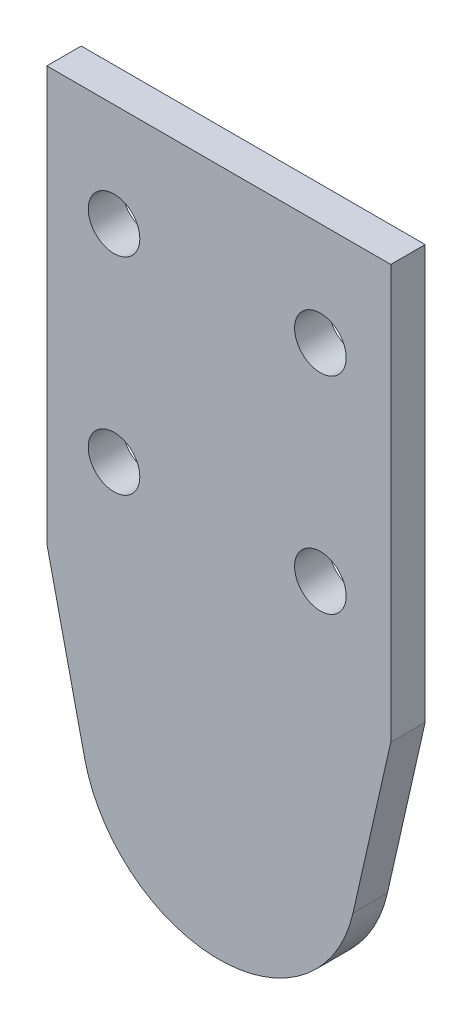
SolidWorks part; units mm, degrees
ref_plane "前视基准面" through (0, 0, 0) normal (0, 0, 1) x (1, 0, 0)
ref_plane "上视基准面" through (0, 0, 0) normal (0, 1, 0) x (1, 0, 0)
ref_plane "右视基准面" through (0, 0, 0) normal (1, 0, 0) x (0, 0, -1)
sketch "草图1" plane through (0, 0, 0) normal (0, 0, 1) x (1, 0, 0)
  line L0 (0, 0) -> (90, 0)
  line L3 (0, 0) -> (5.0194, -161.2446)
  line L4 (90, 0) -> (84.9806, -161.2446)
  arc A0 (5.0194, -161.2446) -> (84.9806, -161.2446) centre (45, -160) ccw
  circle A1 centre (45, -160) radius 20
extrude "凸台-拉伸1" add sketch "草图1" along normal blind 10
sketch "草图2" plane through (0, 0, 10) normal (0, 0, 1) x (1, 0, 0)
  line L0 (0, 0) -> (0, -30)
  line L1 (14.5331, -30) -> (22.0331, -30)
  line L2 (74.5331, -30) -> (74.5331, -90)
  line L3 (74.5331, -90) -> (14.5331, -90)
  line L4 (14.5331, -90) -> (14.5331, -30)
  line L5 (0, -30) -> (22.0331, -30)
  line L6 (84.9806, -161.2446) -> (90, 0) construction
  line L9 (67.0331, -30) -> (74.5331, -30)
  line L10 (67.0331, -30) -> (89.0661, -30)
  circle A0 centre (14.5331, -30) radius 7.5
  circle A1 centre (74.5331, -30) radius 7.5
  circle A2 centre (74.5331, -90) radius 7.5
  circle A3 centre (14.5331, -90) radius 7.5
extrude "切除-拉伸1" cut sketch "草图2" against normal blind 10 contours L1 A0 L5 | L4 A0 L1 | L5 A0 L4 | L10 A1 L9 | L2 A1 L10 | L9 A1 L2 | L3 A2 L2 | L2 A2 L3 | L3 A3 L4 | L4 A3 L3
sketch "草图3" plane through (0, 0, 10) normal (0, 0, 1) x (1, 0, 0)
  line L0 (0, 0) -> (0, -120)
  line L1 (90, 0) -> (90, -120)
  line L2 (90, -120) -> (84.7241, -164.6897)
  line L3 (0, -120) -> (5.2759, -164.6897)
  line L6 (0, 0) -> (5.0194, -161.2446)
  line L7 (0, 0) -> (5.0194, -161.2446)
  line L9 (84.9806, -161.2446) -> (90, 0)
  line L10 (84.9806, -161.2446) -> (90, 0)
  arc A0 (84.7241, -164.6897) -> (5.2759, -164.6897) centre (45, -160) ccw
  line M5 (0, 0) -> (5.0194, -161.2446)
  arc M6 (5.0194, -161.2446) -> (84.9806, -161.2446) centre (45, -160) ccw
  line M7 (84.9806, -161.2446) -> (90, 0)
  dimension "D1" = 0
  dimension "D2" = 0
extrude "凸台-拉伸4" add sketch "草图3" against normal blind 10 contours L2 L1 M7 M6 | L0 L3 M6 M5
sketch "草图4" plane through (0, 0, 0) normal (0, 0, -1) x (-1, 0, 0)
  line L0 (-90, 0) -> (-95, 0)
  line L1 (0, 0) -> (5, 0)
  line L2 (5, 0) -> (5, -120.2941)
  line L3 (-95, 0) -> (-95, -120.2941)
  line L14 (-0.3103, -165.2759) -> (5, -120.2941)
  line L15 (5, -120.2941) -> (5, 5)
  line L16 (5, 5) -> (-95, 5)
  line L17 (-95, 5) -> (-95, -120.2941)
  line L18 (-95, -120.2941) -> (-89.6897, -165.2759)
  line L19 (-95, -120.2941) -> (-84.013, -168.8311)
  line L20 (5, -120.2941) -> (5, 0)
  line L21 (5, -120.2941) -> (-5.987, -168.8311)
  line L22 (-95, 0) -> (-95, -120.2941)
  line L28 (-5.2759, -164.6897) -> (0, -120)
  line L29 (0, -120) -> (0, 0)
  line L30 (0, 0) -> (-90, 0)
  line L31 (-90, 0) -> (-90, -120)
  line L32 (-90, -120) -> (-84.7241, -164.6897)
  line L33 (-5.2759, -164.6897) -> (0, -120)
  line L34 (0, -120) -> (0, 0)
  line L35 (0, 0) -> (-90, 0)
  line L36 (-90, 0) -> (-90, -120)
  line L37 (-90, -120) -> (-84.7241, -164.6897)
  arc A2 (-89.6897, -165.2759) -> (-0.3103, -165.2759) centre (-45, -160) ccw
  arc A3 (-5.987, -168.8311) -> (-5.2759, -164.6897) centre (-45, -160) ccw
  arc A5 (-84.7241, -164.6897) -> (-5.2759, -164.6897) centre (-45, -160) ccw
  arc A6 (-84.7241, -164.6897) -> (-84.013, -168.8311) centre (-45, -160) ccw
  arc M13 (-84.7241, -164.6897) -> (-5.2759, -164.6897) centre (-45, -160) ccw
  line M14 (-5.2759, -164.6897) -> (0, -120)
  line M15 (0, -120) -> (0, 0)
  line M17 (-90, 0) -> (-90, -120)
  line M18 (-90, -120) -> (-84.7241, -164.6897)
  dimension "D1" = 5
  dimension "D2" = 0
extrude "凸台-拉伸8" add sketch "草图4" against normal blind 10 contours L3 L19 L0 M13 M18 M17 | L21 L2 L1 M15 M14 M13
sketch "草图5" plane through (0, 0, 0) normal (0, 0, -1) x (-1, 0, 0)
  circle A1 centre (-45, -160) radius 22.505
extrude "凸台-拉伸9" add sketch "草图5" against normal blind 10
